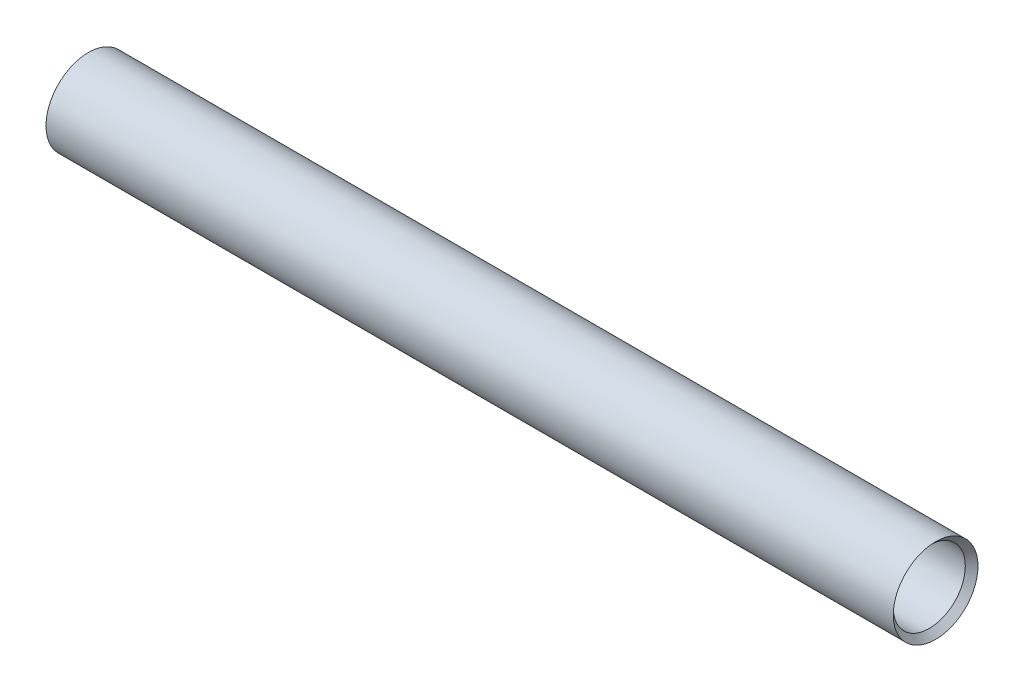
from build123d import *

# Parameters (mm, degrees)
SKETCH1_W                   = 80
SKETCH1_H                   = 4
M8_TAPPED_HOLE1_D           = 6.8
M8_TAPPED_HOLE1_DEPTH       = 18.75
M8_TAPPED_HOLE1_CSINK_D     = 8.05
M8_TAPPED_HOLE1_CSINK_ANGLE = 90
M8_TAPPED_HOLE1_TIP         = 2.042926105


with BuildPart() as part:
    # Sketch1 → Revolve1 (revolve)
    with BuildSketch(Plane.XY, mode=Mode.PRIVATE) as revolve1_sk:
        with Locations((40, 2)):
            Rectangle(SKETCH1_W, SKETCH1_H)
    revolve(revolve1_sk.sketch.rotate(Axis((0, 0, 0), (1, 0, 0)), 90), axis=Axis((0, 0, 0), (1, 0, 0)))

    # M8 Tapped Hole1
    with Locations(Plane(origin=(80, 0, 0), x_dir=(0, 0, 1), z_dir=(1, 0, 0))):
        with Locations((0, 0)):
            CounterSinkHole(M8_TAPPED_HOLE1_D / 2, M8_TAPPED_HOLE1_CSINK_D / 2, depth=M8_TAPPED_HOLE1_DEPTH, counter_sink_angle=M8_TAPPED_HOLE1_CSINK_ANGLE)
            with Locations((0, 0, -(M8_TAPPED_HOLE1_DEPTH + M8_TAPPED_HOLE1_TIP / 2))):  # 118° drill point
                Cone(0, M8_TAPPED_HOLE1_D / 2, M8_TAPPED_HOLE1_TIP, mode=Mode.SUBTRACT)


solid = part.part
